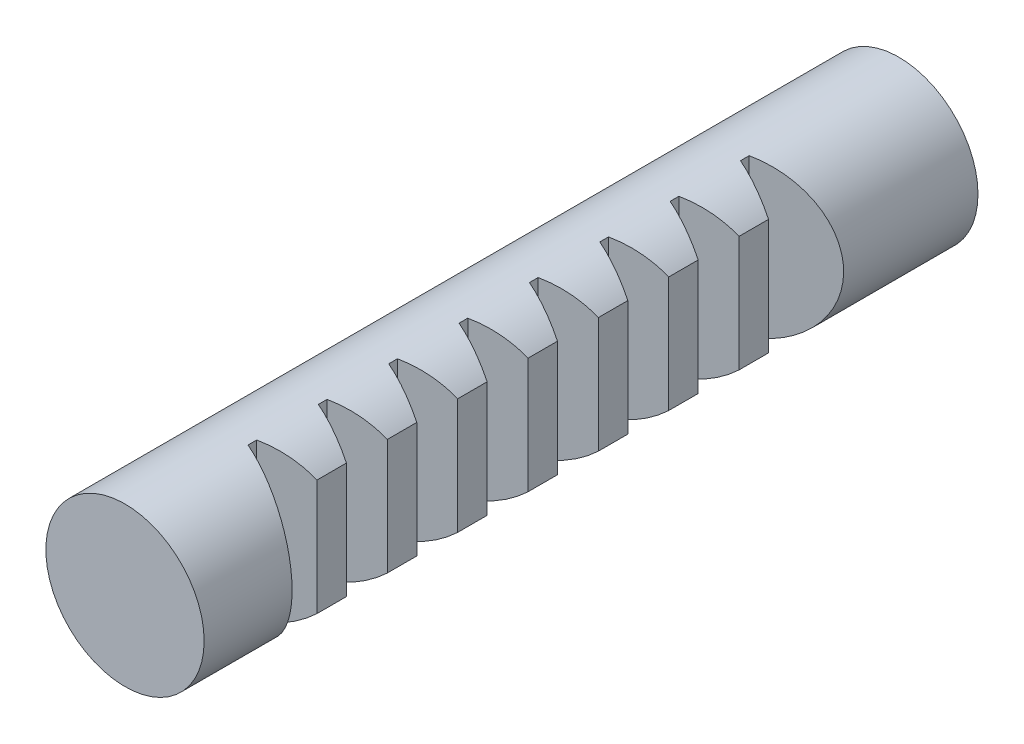
SolidWorks part; units mm, degrees
ref_plane "Front Plane" through (0, 0, 0) normal (0, 0, 1) x (1, 0, 0)
ref_plane "Top Plane" through (0, 0, 0) normal (0, 1, 0) x (1, 0, 0)
ref_plane "Right Plane" through (0, 0, 0) normal (1, 0, 0) x (0, 0, -1)
other "Configuration Table"
sketch "Sketch1" plane through (0, 0, 0) normal (0, 0, 1) x (1, 0, 0)
  circle A0 centre (0, 0) radius 9
  dimension "D1" = 18
extrude "Boss-Extrude1" add sketch "Sketch1" along normal mid plane 88
sketch "Sketch2" plane through (0, 0, 0) normal (0, 1, 0) x (1, 0, 0)
  line L0 (9, -34) -> (1.125, -31.1337)
  line L1 (9, -44) -> (9, 44) construction
  line L2 (-9, -44) -> (9, -44) construction
  line L3 (1.125, -31.1337) -> (1.125, -30.1436)
  line L4 (1.125, -30.6387) -> (14.6168, -30.6387) construction
  line L5 (9, -34) -> (9, -27.2774)
  line L6 (3, -31.8162) -> (3, -29.4612) construction
  line L7 (9, -27.2774) -> (1.125, -30.1436)
  point P15 (3, -30.6387)
  point P16 (9, -30.6387)
  dimension "D1" = 10
  dimension "D2" = 2.355
  dimension "D3" = 1.875
  dimension "D4" = 20
  dimension "D5" = 3
extrude "Cut-Extrude1" cut sketch "Sketch2" against normal through all both and the other way through all
sketch "Sketch3" plane through (0, 0, 0) normal (0, 1, 0) x (1, 0, 0)
  line L0 (-11.5594, -10.3586) -> (-11.5594, 10.2008) construction
pattern_linear "LPattern1" count 8 spacing 8 along (0, 0, -1) of "Cut-Extrude1"
sketch "Sketch4" plane through (0, 0, 0) normal (0, 1, 0) x (1, 0, 0)
  line L1 (6.1419, 26.6844) -> (17.2459, 26.6844)
  line L2 (6.1419, 26.6844) -> (6.1419, -29.0785)
  line L3 (6.1419, -29.0785) -> (17.2459, -29.0785)
  line L4 (17.2459, 26.6844) -> (17.2459, -29.0785)
  line L5 (6.1419, 26.6844) -> (17.2459, -29.0785) construction
  line L6 (6.1419, -29.0785) -> (17.2459, 26.6844) construction
  point P0 (11.6939, -1.1971)
extrude "Cut-Extrude2" cut sketch "Sketch4" against normal through all both and the other way through all
